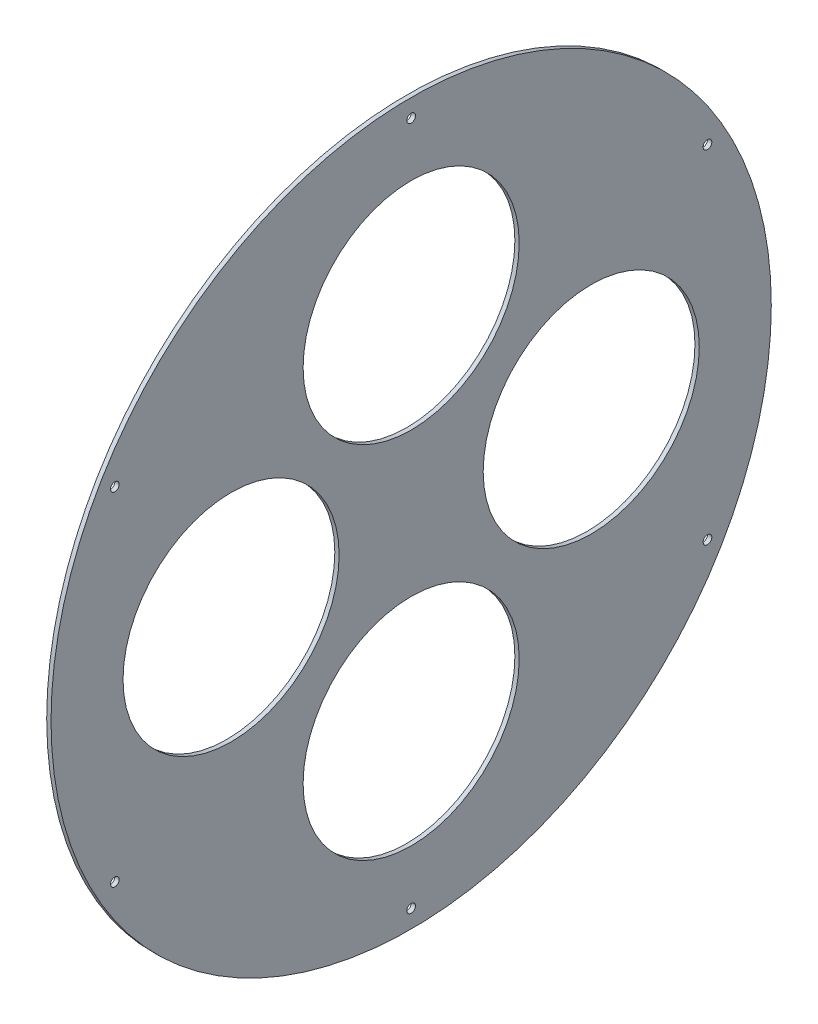
SolidWorks part; units mm, degrees
material "AISI 304"
ref_plane "Front Plane" through (0, 0, 0) normal (0, 0, 1) x (1, 0, 0)
ref_plane "Top Plane" through (0, 0, 0) normal (0, 1, 0) x (1, 0, 0)
ref_plane "Right Plane" through (0, 0, 0) normal (1, 0, 0) x (0, 0, -1)
sketch "Sketch1" plane through (0, 0, 0) normal (1, 0, 0) x (0, 0, -1)
  circle A0 centre (0, 0) radius 250
  dimension "D1" = 500
extrude "Boss-Extrude1" add sketch "Sketch1" along normal blind 3
sketch "Sketch2" plane through (3, 0, 0) normal (1, 0, 0) x (0, 0, -1)
  line L0 (0, 0) -> (0, 250) construction
  circle A0 centre (0, 125) radius 75
  dimension "D1" = 125
  dimension "D2" = 150
extrude "Cut-Extrude1" cut sketch "Sketch2" against normal blind 10
pattern_circular "CirPattern1" count 4 every 90 about axis through (0, 0, 0) along (1, 0, 0) of "Cut-Extrude1"
sketch "Sketch3" plane through (3, 0, 0) normal (1, 0, 0) x (0, 0, -1)
  line L0 (0, 0) -> (0, -312.4202) construction
  circle A0 centre (0, -237.5) radius 3
  dimension "D1" = 6
  dimension "D2" = 237.5
extrude "Cut-Extrude2" cut sketch "Sketch3" against normal blind 20
pattern_circular "CirPattern2" count 6 over 360 about axis through (0, 0, 0) along (1, 0, 0) of "Cut-Extrude2"
